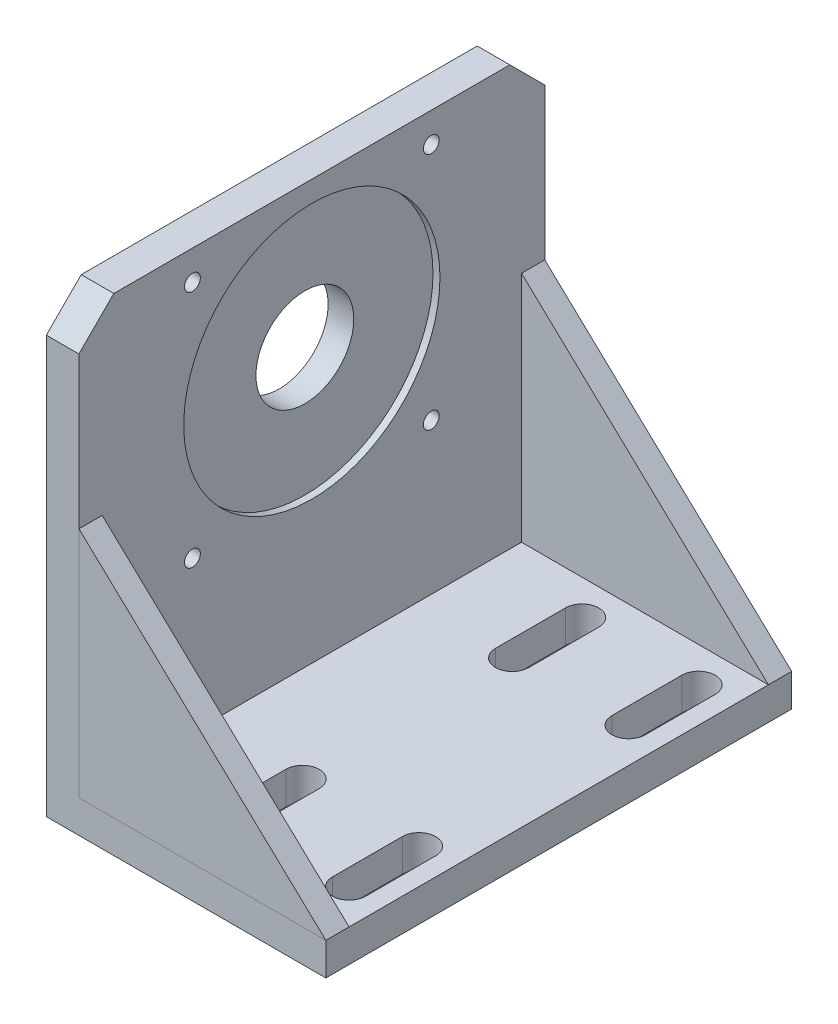
from build123d import *

# Parameters (mm, degrees)
SKETCH_1_W               = 120
SKETCH_1_H               = 200
EXTRUDE_1_DEPTH          = 14
SKETCH_2_W               = 14
SKETCH_2_H               = 200
EXTRUDE_2_DEPTH          = 180
EXTRUDE_3_DEPTH          = 10
EXTRUDE_4_DEPTH          = 10
SKETCH_5_R               = 21
CUT_EXTRUDE_1_DEPTH      = 12
SKETCH_6_R               = 15
CUT_EXTRUDE_2_DEPTH      = 244.515913238
SKETCH_7_R               = 55
CUT_EXTRUDE_3_DEPTH      = 3
CUT_EXTRUDE_4_DEPTH      = 215.476105895
SKETCH_10_W              = 3.4
SKETCH_10_H              = 14
PATTERN_CIRCULAR_1_COUNT = 4
CHAMFER_1_SIZE           = 15


with BuildPart() as part:
    # 草图1 → 凸台-拉伸1 (new body)
    with BuildSketch(Plane(origin=(0, 0, 0), x_dir=(1, 0, 0), z_dir=(0, 1, 0))):
        Rectangle(SKETCH_1_W, SKETCH_1_H)
    extrude(amount=EXTRUDE_1_DEPTH)

    # 草图2 → 凸台-拉伸2 (add)
    with BuildSketch(Plane(origin=(0, 14, 0), x_dir=(1, 0, 0), z_dir=(0, 1, 0))):
        with Locations((-53, 0)):
            Rectangle(SKETCH_2_W, SKETCH_2_H)
    extrude(amount=EXTRUDE_2_DEPTH)

    # 草图5 → 切除-拉伸1 (cut)
    with BuildSketch(Plane.ZY.offset(60)):
        with Locations((0, 130)):
            Circle(SKETCH_5_R)
    extrude(amount=-CUT_EXTRUDE_1_DEPTH, mode=Mode.SUBTRACT)

    # 草图6 → 切除-拉伸2 (cut, through all)
    with BuildSketch(Plane.ZY.offset(48)):
        with Locations((0, 130)):
            Circle(SKETCH_6_R)
    extrude(amount=-CUT_EXTRUDE_2_DEPTH, mode=Mode.SUBTRACT)

    # 草图7 → 切除-拉伸3 (cut)
    with BuildSketch(Plane(origin=(-46, 0, 0), x_dir=(0, 0, -1), z_dir=(1, 0, 0))):
        with Locations((0, 130)):
            Circle(SKETCH_7_R)
    extrude(amount=-CUT_EXTRUDE_3_DEPTH, mode=Mode.SUBTRACT)

    # 草图8 → 切除-拉伸4 (cut, through all)
    with BuildSketch(Plane(origin=(0, 14, 0), x_dir=(1, 0, 0), z_dir=(0, 1, 0))):
        with BuildLine():
            Line((2.166144886, 75), (2.166144886, 45))
            ThreePointArc((2.166144886, 45), (-5, 37.833855114), (-12.166144886, 45))
            Line((-12.166144886, 45), (-12.166144886, 75))
            ThreePointArc((-12.166144886, 75), (-5, 82.166144886), (2.166144886, 75))
        make_face()
        with BuildLine():
            Line((52.166144886, 75), (52.166144886, 45))
            ThreePointArc((52.166144886, 45), (45, 37.833855114), (37.833855114, 45))
            Line((37.833855114, 45), (37.833855114, 75))
            ThreePointArc((37.833855114, 75), (45, 82.166144886), (52.166144886, 75))
        make_face()
        with BuildLine():
            Line((2.166144886, -75), (2.166144886, -45))
            ThreePointArc((2.166144886, -45), (-5, -37.833855114), (-12.166144886, -45))
            Line((-12.166144886, -45), (-12.166144886, -75))
            ThreePointArc((-12.166144886, -75), (-5, -82.166144886), (2.166144886, -75))
        make_face()
        with BuildLine():
            Line((52.166144886, -75), (52.166144886, -45))
            ThreePointArc((52.166144886, -45), (45, -37.833855114), (37.833855114, -45))
            Line((37.833855114, -45), (37.833855114, -75))
            ThreePointArc((37.833855114, -75), (45, -82.166144886), (52.166144886, -75))
        make_face()
    extrude(amount=-CUT_EXTRUDE_4_DEPTH, mode=Mode.SUBTRACT)

    # 草图10 → M8 螺纹孔1 (revolve, cut)
    with BuildSketch(Plane(origin=(-46, 181.265241636, 51.265241636), x_dir=(0, 0, -1), z_dir=(0, 1, 0))):
        with Locations((1.7, 7)):
            Rectangle(SKETCH_10_W, SKETCH_10_H)
    hole_wizard_m8_1 = revolve(axis=Axis((-39.65, 181.265241636, 51.265241636), (-1, 0, 0)), mode=Mode.SUBTRACT)

    # 阵列(圆周)1: M8 螺纹孔1 ×4 about axis
    pattern_circular_1_axis = Axis((0, 130, 0), (1, 0, 0))
    for i in range(1, PATTERN_CIRCULAR_1_COUNT):
        add(hole_wizard_m8_1.rotate(pattern_circular_1_axis, i * 360 / PATTERN_CIRCULAR_1_COUNT), mode=Mode.SUBTRACT)

    # 倒角1
    chamfer_1_edges = [part.edges().sort_by_distance(p)[0] for p in [
        (-53, 194, 100),
        (-53, 194, -100),
    ]]
    chamfer(chamfer_1_edges, length=CHAMFER_1_SIZE)


with BuildPart() as body_2:
    # 草图3 → 凸台-拉伸3 (new body)
    with BuildSketch(Plane.XY.offset(100)):
        Polygon((-46, 114), (60, 14), (-46, 14), align=None)
    extrude(amount=-EXTRUDE_3_DEPTH)


with BuildPart() as body_3:
    # 草图4 → 凸台-拉伸4 (new body)
    with BuildSketch(Plane(origin=(0, 0, -100), x_dir=(-1, 0, 0), z_dir=(0, 0, -1))):
        Polygon((46, 14), (46, 114), (-60, 14), align=None)
    extrude(amount=-EXTRUDE_4_DEPTH)


solid = Compound([part.part, body_2.part, body_3.part])
